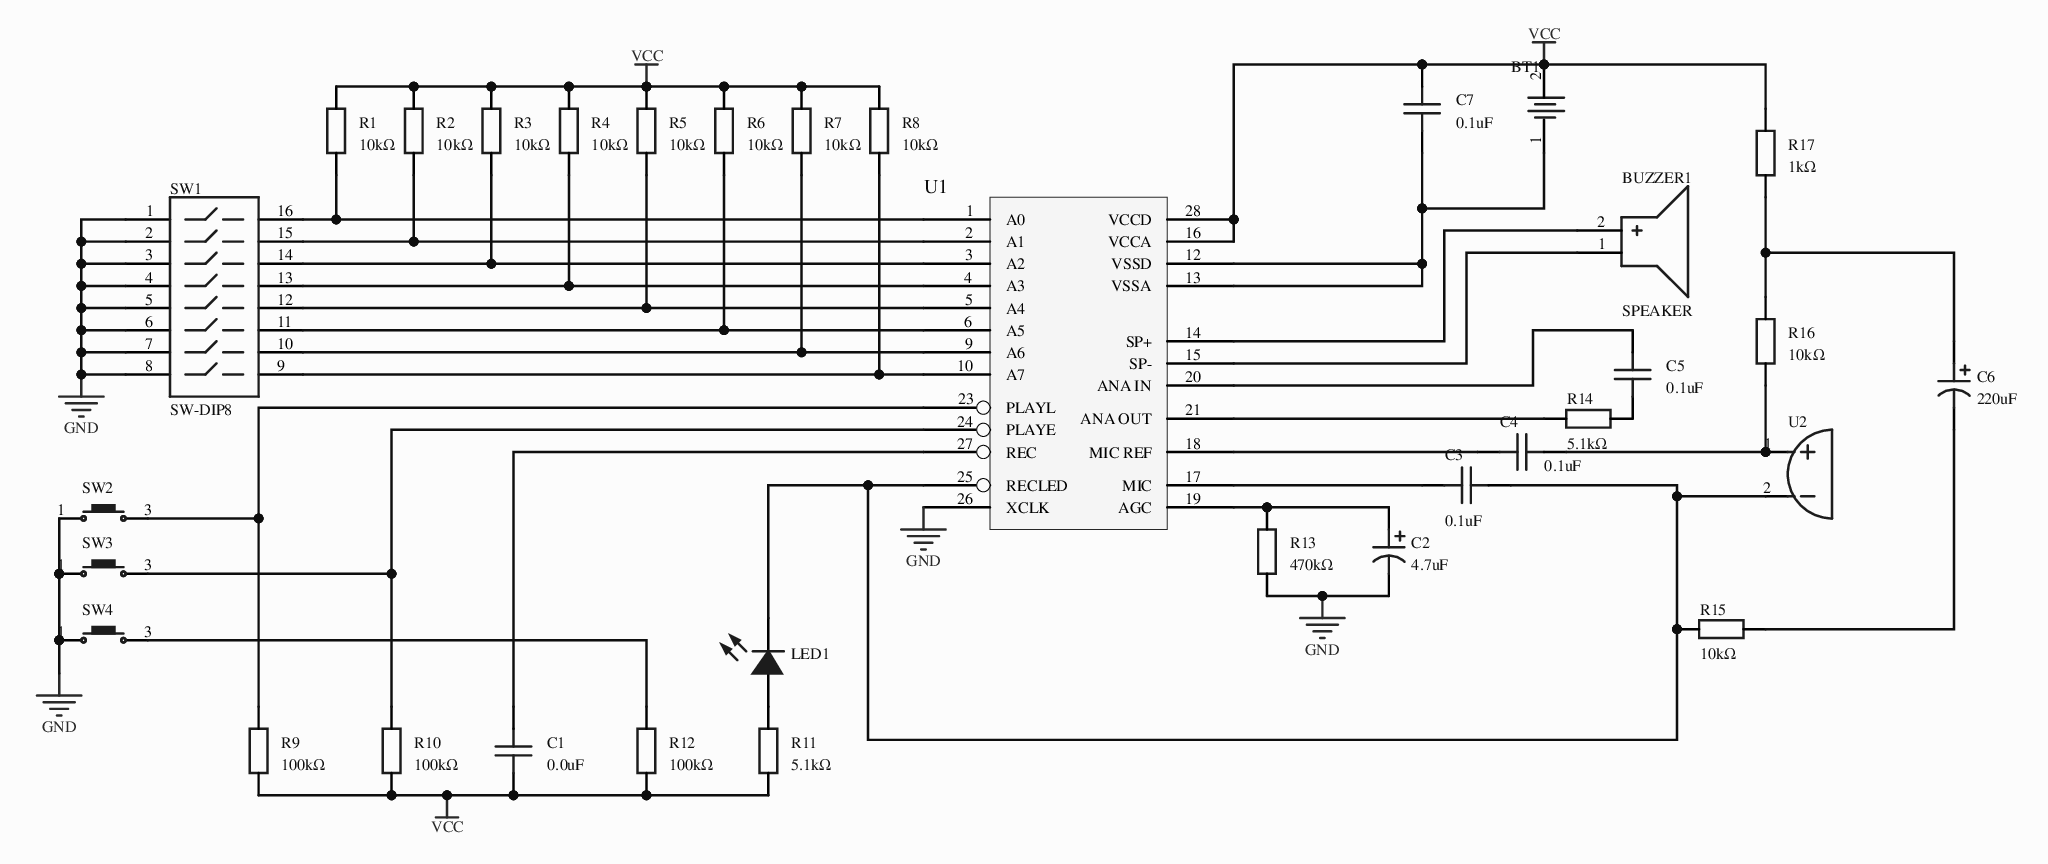
[diagram p0: MISC51898-3.schdoc]
# Altium project MISC51898.PrjPcb
1 sheet, 33 parts. Net scope: global (net labels, ports and power ports of the same name join across sheets).
Board file: MISC51898.pcbdoc

## Sheet MISC51898-3.schdoc
size 297 x 209 mm; Version: V1.0; @Project Name: MISC51898; @Update Date: 2026-09-23; @Create Date: 2026-09-23; @Board Name: MISC51898; @Create Time: 13:48:54; @Page Count: 1; @Page No: 1; @Schematic Name: MISC51898; @Update Time: 13:48:54; Size: A4

### Parts
BT1  (no value)  [HDR-TH_2P-P2.54-V-M-1]
BUZZER1  SPEAKER  [BUZ-TH_BD12.0-P6.00-D0.9-RD]
C1  0.0uF  [CAP-TH_L5.1-W3.2-P5.08-D0.50]
C2  4.7uF  [CAP-TH_BD5.0-P2.00-D0.8-FD-10UF50VC110GL]
C3  0.1uF  [CAP-TH_L5.1-W3.2-P5.08-D0.50]
C4  0.1uF  [CAP-TH_L5.1-W3.2-P5.08-D0.50]
C5  0.1uF  [CAP-TH_L5.1-W3.2-P5.08-D0.50]
C6  220uF  [CAP-TH_BD5.0-P2.00-D0.8-FD-10UF50VC110GL]
C7  0.1uF  [CAP-TH_L5.1-W3.2-P5.08-D0.50]
LED1  (no value)  [LED_TH-3mm]
R1  10kΩ  [Res_1/4W]
R2  10kΩ  [Res_1/4W]
R3  10kΩ  [Res_1/4W]
R4  10kΩ  [Res_1/4W]
R5  10kΩ  [Res_1/4W]
R6  10kΩ  [Res_1/4W]
R7  10kΩ  [Res_1/4W]
R8  10kΩ  [Res_1/4W]
R9  100kΩ  [Res_1/8W]
R10  100kΩ  [Res_1/8W]
R11  5.1kΩ  [Res_1/8W]
R12  100kΩ  [Res_1/8W]
R13  470kΩ  [Res_1/4W]
R14  5.1kΩ  [Res_1/4W]
R15  10kΩ  [Res_1/4W]
R16  10kΩ  [Res_1/4W]
R17  1kΩ  [Res_1/4W]
SW1  SW-DIP8  [SW-DIP8]
SW2  (no value)  [SW-TH_4P-L6.0-W6.0-P4.50-LS6.5]
SW3  (no value)  [SW-TH_4P-L6.0-W6.0-P4.50-LS6.5]
SW4  (no value)  [SW-TH_4P-L6.0-W6.0-P4.50-LS6.5]
U1  (no value)
U2  (no value)

### Nets
GND: C2.2 R13.1 SW1.1 SW1.2 SW1.3 SW1.4 SW1.5 SW1.6 SW1.7 SW1.8 SW2.1 SW3.1 SW4.1 U1.26(XCLK)
VCC: BT1.2 C1.1 C7.2 R1.2 R2.2 R3.2 R4.2 R5.2 R6.2 R7.2 R8.2 R9.1 R10.1 R11.1 R12.1 R17.2 U1.16(VCCA) U1.28(VCCD)
NetBT1_1: BT1.1 C7.1 U1.12(VSSD) U1.13(VSSA)
NetBUZZER1_1: BUZZER1.1(-) U1.15(SP-)
NetBUZZER1_2: BUZZER1.2(+) U1.14(SP+)
NetC1_2: C1.2 U1.27(REC)
NetC2_1: C2.1 R13.2 U1.19(AGC)
NetC3_1: C3.1 U1.17(MIC)
NetC3_2: C3.2 LED1.2(A) R15.1 U1.25(RECLED) U2.2
NetC4_1: C4.1 U1.18(MIC_REF)
NetC4_2: C4.2 R16.1 U2.1
NetC5_1: C5.1 R14.1
NetC5_2: C5.2 U1.20(ANA_IN)
NetC6_1: C6.1 R16.2 R17.1
NetC6_2: C6.2 R15.2
NetLED1_1: LED1.1(C) R11.2
NetR1_1: R1.1 SW1.16 U1.1(A0)
NetR2_1: R2.1 SW1.15 U1.2(A1)
NetR3_1: R3.1 SW1.14 U1.3(A2)
NetR4_1: R4.1 SW1.13 U1.4(A3)
NetR5_1: R5.1 SW1.12 U1.5(A4)
NetR6_1: R6.1 SW1.11 U1.6(A5)
NetR7_1: R7.1 SW1.10 U1.9(A6)
NetR8_1: R8.1 SW1.9 U1.10(A7)
NetR9_2: R9.2 SW2.3 U1.23(PLAYL)
NetR10_2: R10.2 SW3.3 U1.24(PLAYE)
NetR12_2: R12.2 SW4.3
NetR14_2: R14.2 U1.21(ANA_OUT)

### Library data of the parts
BT1 = HDR-M_2.54_1x2P: Symbol: 210S-1*2P L=11.6MMGold-plated black; ConvertToPcb: yes; ModelId: 79b2e9f2d70a4d68a1b7098f27c6d4c50819f05c4eef4c71ace90d822a990e87; ModelName: HDR-M-2.54_1x2; ModelTransform: 200,100,0,0,0,0,0,0,-118.11; Device: HDR-M_2.54_1x2P; FootprintName: HDR-TH_2P-P2.54-V-M-1; AddInBom: yes; SupplierPart: C124375; Supplier Footprint: 插件
BUZZER1 = buzzer: AddInBom: yes; ModelId: af17e4151ed84fc2a628230bf23763630819f05c4eef4c71ace90d822a990e87; ModelTransform: 472.44,472.176,0,270,0,0,0,0,-196.85; Symbol: BUZZER; Device: buzzer; Manufacturer Part: SPEAKER; LCSC Part Name: buzzer; SupplierPart: C9900014030; Supplier Footprint: buzzer; JLCPCB Part Class: Extended Part; Supplier: LCSC; ConvertToPcb: yes; FootprintName: BUZ-TH_BD12.0-P6.00-D0.9-RD; ModelName: BUZ-TH_BD12.0-P6.00-D0.9-RD
C1 = C323C104K5R5TA7301: Capacitance:100nF;Tolerance:±10%;Rated voltage:50V;Temperature coefficient:X7R;; Manufacturer: KEMET(基美); AddInBom: yes; ModelId: 5e578892460b443ea6286c5f4e214fbb0819f05c4eef4c71ace90d822a990e87; ModelTransform: 219.6846,125.5903,0,0,0,0,0,0,-196.85; Tolerance: ±10%; Voltage Rating: 50V; Temperature Coefficient: X7R; Pin Spacing: 5.08mm; Symbol: C323C104K5R5TA7301; Device: C323C104K5R5TA7301; Value: 0.0uF; FootprintName: CAP-TH_L5.1-W3.2-P5.08-D0.50; LCSC Part Name: 100nF ±10% 50V; ManufacturerPart: C323C104K5R5TA7301; Supplier Footprint: 插件,P=5.08mm; JLCPCB Part Class: Extended Part; Datasheet: https://item.szlcsc.com/datasheet/C323C104K5R5TA7301/194969.html; Supplier: LCSC; ConvertToPcb: yes; ModelName: CAP-TH_L5.1-W3.2-P5.08-D0.50
C2 C6 = 10UF50VC110GL: Capacitance:10uF;Tolerance:±20%;Rated voltage:50V;Ripple current:120mA@100KHz;Equivalent series resistance(ESR):1.6Ω;; Manufacturer: Econd(米朗电子); AddInBom: yes; ModelId: b35ab6b0460c4c43a629d91cfc2b58780819f05c4eef4c71ace90d822a990e87; ModelTransform: 196.85,196.85,0,0,0,0,0,0,-196.85; Tolerance: ±20%; Voltage Rating: 50V; Equivalent Series Resistance(ESR): 1.6Ω; Pin Spacing: 2mm; Lifetime: 5000hrs@105℃; Symbol: 10UF50VC110GL; Device: 10UF50VC110GL; FootprintName: CAP-TH_BD5.0-P2.00-D0.8-FD-10UF50VC110GL; LCSC Part Name: 10uF ±20% 50V; ManufacturerPart: 10UF50VC110GL; Supplier Footprint: 插件,D5xL11mm; JLCPCB Part Class: Extended Part; Datasheet: https://item.szlcsc.com/datasheet/10UF50VC110GL/49031974.html; Supplier: LCSC; ConvertToPcb: yes; ModelName: CAP-TH_BD5.0-P2.00-D0.8-FD-10UF50VC110GL; Ripple Current: 120mA@100KHz; Diameter: 5mm; Height - Seated (Max): 11mm; Operating Temperature: -40℃~+105℃
  C2: Value: 4.7uF
  C6: Value: 220uF
C3-C5 C7 = C323C104K5R5TA7301: Capacitance:100nF;Tolerance:±10%;Rated voltage:50V;Temperature coefficient:X7R;; Manufacturer: KEMET(基美); 3D Model: 5e578892460b443ea6286c5f4e214fbb0819f05c4eef4c71ace90d822a990e87; 3D Model Transform: 219.6846,125.5903,0,0,0,0,0,0,-196.85; Tolerance: ±10%; Voltage Rating: 50V; Temperature Coefficient: X7R; Pin Spacing: 5.08mm; AddInBom: yes; Symbol: C323C104K5R5TA7301; Device: C323C104K5R5TA7301; LCSC Part Name: 100nF ±10% 50V; Manufacturer Part: C323C104K5R5TA7301; Supplier Footprint: 插件,P=5.08mm; JLCPCB Part Class: Extended Part; Datasheet: https://item.szlcsc.com/datasheet/C323C104K5R5TA7301/194969.html; Supplier: LCSC; Value: 0.1uF; FootprintName: CAP-TH_L5.1-W3.2-P5.08-D0.50; ConvertToPcb: yes; ModelName: CAP-TH_L5.1-W3.2-P5.08-D0.50
LED1 = LED_TH-B_3mm: ConvertToPcb: yes; ModelId: ff771fff7070432ca3f353cf0f67af4c0819f05c4eef4c71ace90d822a990e87; ModelName: LED-TH_BD3.8-P2.54-FD_BLUE; ModelTransform: 134.36,149.37,405.47,0,0,0,-11.81,0,-196.85; Symbol: LED_TH-B; Device: LED_TH-B_3mm; FootprintName: LED_TH-3mm; AddInBom: yes; Supplier Footprint: 插件
R1-R8 = Res_AXIAL-1/4W: Symbol: resistor; AddInBom: yes; ModelId: 463263665006444ab7a47bd11b0cf9560819f05c4eef4c71ace90d822a990e87; ModelName: RES-TH_BD2.4-L6.3-P10.30-D0.6; ModelTransform: 427.165,94.32816,0,0,0,0,0,0,-196.85; Device: Res_AXIAL-1/4W; FootprintName: Res_1/4W; Supplier Footprint: 轴向引线; ConvertToPcb: yes; Value: 10kΩ
R9-R11 = Res_AXIAL-1/8W: Symbol: resistor; ConvertToPcb: yes; ModelId: b2b5ae7ae4c642178fe0039925c86a3f0819f05c4eef4c71ace90d822a990e87; ModelName: RES-TH_BD1.8-L3.2-P7.20-D0.4; ModelTransform: 282.86,66.88,253.09,0,0,0,0,0,-191; Device: Res_AXIAL-1/8W; FootprintName: Res_1/8W; AddInBom: yes; Supplier Footprint: 轴向引线
  R9 R10: Value: 100kΩ
  R11: Value: 5.1kΩ
R12 = Res_AXIAL-1/8W: Symbol: resistor; 3D Model: b2b5ae7ae4c642178fe0039925c86a3f0819f05c4eef4c71ace90d822a990e87; 3D Model Transform: 282.86,66.88,253.09,0,0,0,0,0,-191; ConvertToPcb: yes; ModelName: RES-TH_BD1.8-L3.2-P7.20-D0.4; Device: Res_AXIAL-1/8W; Value: 100kΩ; Supplier Footprint: 轴向引线; FootprintName: Res_1/8W; AddInBom: yes
R13-R17 = Res_AXIAL-1/4W: Symbol: resistor; 3D Model: 463263665006444ab7a47bd11b0cf9560819f05c4eef4c71ace90d822a990e87; 3D Model Transform: 427.165,94.32816,0,0,0,0,0,0,-196.85; AddInBom: yes; ModelName: RES-TH_BD2.4-L6.3-P10.30-D0.6; Device: Res_AXIAL-1/4W; Supplier Footprint: 轴向引线; FootprintName: Res_1/4W; ConvertToPcb: yes
  R13: Value: 470kΩ
  R14: Value: 5.1kΩ
  R15 R16: Value: 10kΩ
  R17: Value: 1kΩ
SW1 = SW-DIP8: AddInBom: yes; Symbol: SW-DIP8; Device: SW-DIP8; FootprintName: SW-DIP8; Published: 24-Mar-1999; LatestRevisionDate: 17-Dec-2003; LatestRevisionNote: PCB Footprint replaced.; PackageReference: DIP-16-KEY; ComponentLink1Description: Manufacturer Link; ConvertToPcb: yes; Publisher: Altium Limited
SW2-SW4 = Key_TH_6x6x6: Contact current:50mA;Rated voltage(DC):12V;Insulation resistance:100MΩ;Circuit structure:SPST;Mounting:through-hole;Button shape:round button;Button/cap colour:black;Actuation force:260gf@±30gf;Operating temperature:-25℃~+70℃;Pin style:PC pin;Switch length:6mm;Switch width:6mm;Switch height:6mm;With bracket:no;; Symbol: tactile key; AddInBom: yes; ModelId: 20eee248bc684ccd8cbdbb1d0d91ec6f0819f05c4eef4c71ace90d822a990e87; ModelName: SW-TH_4P-L6.0-W6.0-H5.0-LS6.5-P4.50; ModelTransform: 236.22,323.03,0,90,0,0,0,0,-137.795; Device: Key_TH_6x6x6; FootprintName: SW-TH_4P-L6.0-W6.0-P4.50-LS6.5; ConvertToPcb: yes; Supplier Footprint: 插件
U1 = ISD1400: ConvertToPcb: yes; Symbol: ISD1400; Device: ISD1400; AddInBom: yes
U2 = 咪头: Symbol: microphone capsule; AddInBom: yes; Device: microphone capsule; ConvertToPcb: yes